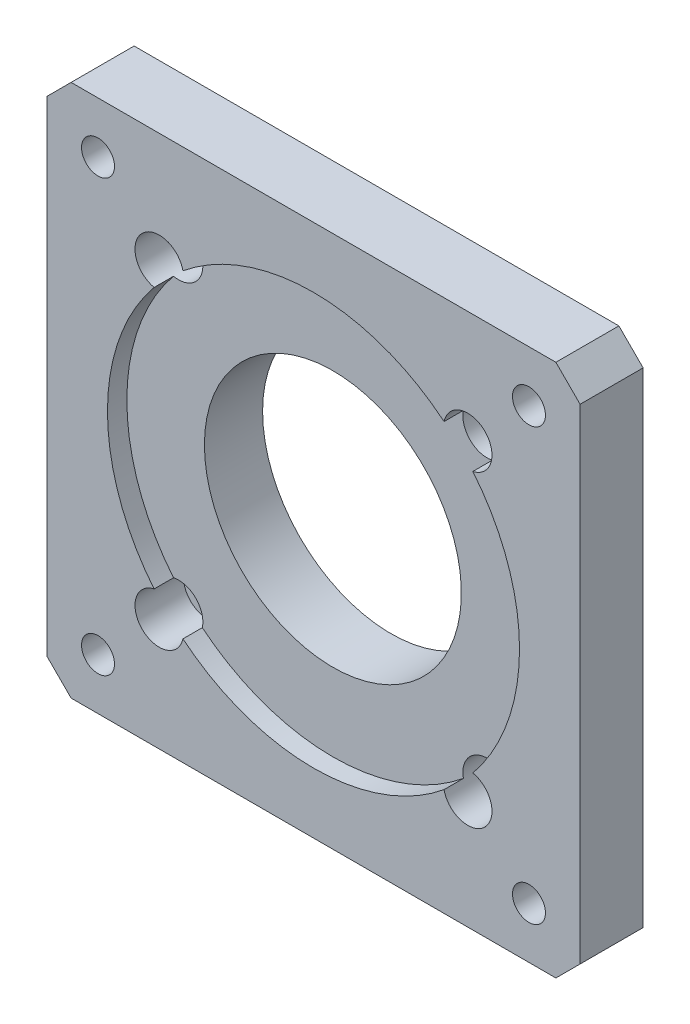
from build123d import *

# Parameters (mm, degrees)
SKETCH_1_W                   = 110
SKETCH_1_H                   = 110
EXTRUDE_1_DEPTH              = 13
SKETCH_2_R                   = 42.5
CUT_EXTRUDE_1_DEPTH          = 4
SKETCH_3_R                   = 26.5
CUT_EXTRUDE_2_DEPTH          = 79.860636569
EXTRUDE_START                = 3
SKETCH_4_R                   = 35
SKETCH_4_R_2                 = 26.5
EXTRUDE_2_DEPTH              = 3
HOLE_WIZARD_M8_1_D           = 6.8
CHAMFER_1_SIZE               = 5
HOLE_WIZARD_M5_1_D           = 5.8
HOLE_WIZARD_M5_1_CBORE_D     = 10
HOLE_WIZARD_M5_1_CBORE_DEPTH = 10
CHAMFER_2_SIZE               = 0.5


with BuildPart() as part:
    # 草图1 → 凸台-拉伸1 (new body)
    with BuildSketch(Plane.XY):
        Rectangle(SKETCH_1_W, SKETCH_1_H)
    extrude(amount=EXTRUDE_1_DEPTH)

    # 草图2 → 切除-拉伸1 (cut)
    with BuildSketch(Plane.XY.offset(13)):
        Circle(SKETCH_2_R)
    extrude(amount=-CUT_EXTRUDE_1_DEPTH, mode=Mode.SUBTRACT)

    # 草图3 → 切除-拉伸2 (cut, through all)
    with BuildSketch(Plane(origin=(0, 0, 0), x_dir=(-1, 0, 0), z_dir=(0, 0, -1))):
        Circle(SKETCH_3_R)
    extrude(amount=-CUT_EXTRUDE_2_DEPTH, mode=Mode.SUBTRACT)

    # 草图4 → 凸台-拉伸2 (add)
    with BuildSketch(Plane(origin=(0, 0, 0), x_dir=(-1, 0, 0), z_dir=(0, 0, -1)).offset(EXTRUDE_START)):
        with Locations(Location((0, 0, 0), (0, 0, 180))):
            Circle(SKETCH_4_R)
        Circle(SKETCH_4_R_2, mode=Mode.SUBTRACT)
    extrude(amount=-EXTRUDE_2_DEPTH)

    # M8 螺纹孔1 (through all)
    with Locations(Plane(origin=(0, 0, 0), x_dir=(-1, 0, 0), z_dir=(0, 0, -1))):
        with Locations((-44.45, 44.45), (44.45, 44.45), (44.45, -44.45), (-44.45, -44.45)):
            Hole(HOLE_WIZARD_M8_1_D / 2)

    # 倒角1
    chamfer_1_edges = [part.edges().sort_by_distance(p)[0] for p in [
        (55, -55, 6.5),
        (-55, -55, 6.5),
        (-55, 55, 6.5),
        (55, 55, 6.5),
    ]]
    chamfer(chamfer_1_edges, length=CHAMFER_1_SIZE)

    # M5 六角凹头螺钉的柱形沉头孔1 (through all)
    with Locations(Plane.XY.offset(13)):
        with Locations((-31.819805153, 31.819805153), (-31.819805153, -31.819805153), (31.819805153, -31.819805153), (31.819805153, 31.819805153)):
            CounterBoreHole(HOLE_WIZARD_M5_1_D / 2, HOLE_WIZARD_M5_1_CBORE_D / 2, HOLE_WIZARD_M5_1_CBORE_DEPTH)

    # 倒角2
    chamfer_2_edges = [part.edges().sort_by_distance(p)[0] for p in [
        (-35, 0, -3),
    ]]
    chamfer(chamfer_2_edges, length=CHAMFER_2_SIZE)


solid = part.part
